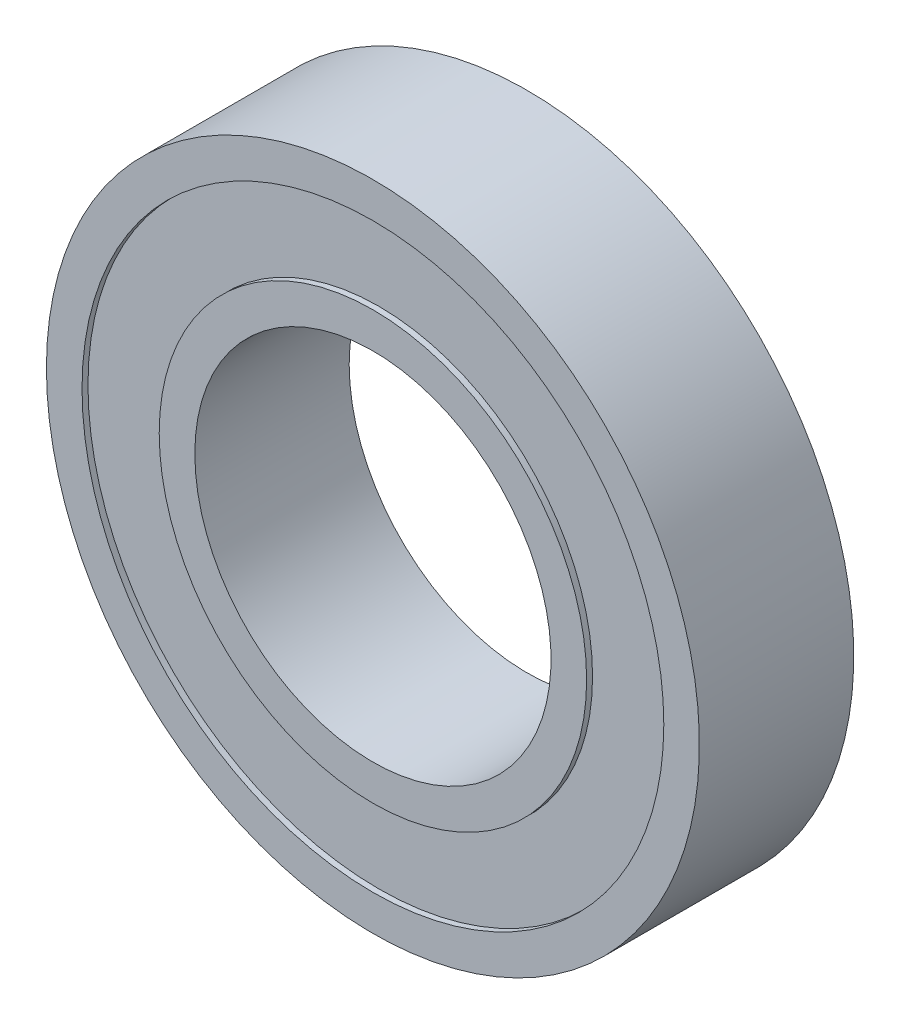
from build123d import *

# Parameters (mm, degrees)
SKETCH1_R           = 27.5
SKETCH1_R_2         = 15
BOSS_EXTRUDE1_DEPTH = 6.5
SKETCH2_R           = 24.5
SKETCH2_R_2         = 18
CUT_EXTRUDE1_DEPTH  = 0.5


with BuildPart() as part:
    # Sketch1 → Boss-Extrude1 (new, symmetric)
    with BuildSketch(Plane.XY):
        with Locations(Location((0, 0, 0), (0, 0, 180))):
            Circle(SKETCH1_R)
        with Locations(Location((0, 0, 0), (0, 0, 180))):
            Circle(SKETCH1_R_2, mode=Mode.SUBTRACT)
    extrude(amount=BOSS_EXTRUDE1_DEPTH, both=True)

    # Sketch2 → Cut-Extrude1 (cut)
    with BuildSketch(Plane.XY.offset(6.5)):
        Circle(SKETCH2_R)
        Circle(SKETCH2_R_2, mode=Mode.SUBTRACT)
    cut_extrude1 = extrude(amount=-CUT_EXTRUDE1_DEPTH, mode=Mode.SUBTRACT)

    # Mirror1: Cut-Extrude1 across plane
    add(cut_extrude1.mirror(Plane.XY), mode=Mode.SUBTRACT)


solid = part.part
